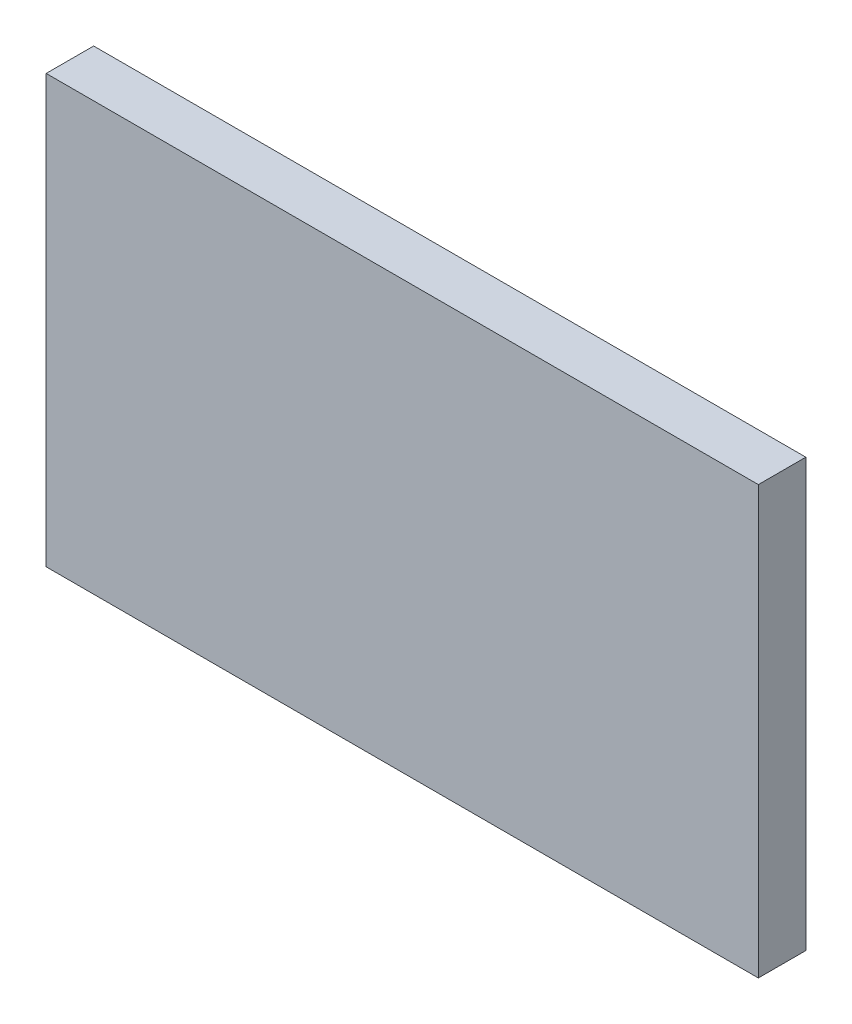
from build123d import *

# Parameters (mm, degrees)
SKETCH_1_W      = 150
SKETCH_1_H      = 90
EXTRUDE_1_DEPTH = 10


with BuildPart() as part:
    # 草图1 → 凸台-拉伸1 (new body)
    with BuildSketch(Plane.XY):
        with Locations((75, 45)):
            Rectangle(SKETCH_1_W, SKETCH_1_H)
    extrude(amount=EXTRUDE_1_DEPTH)


solid = part.part
